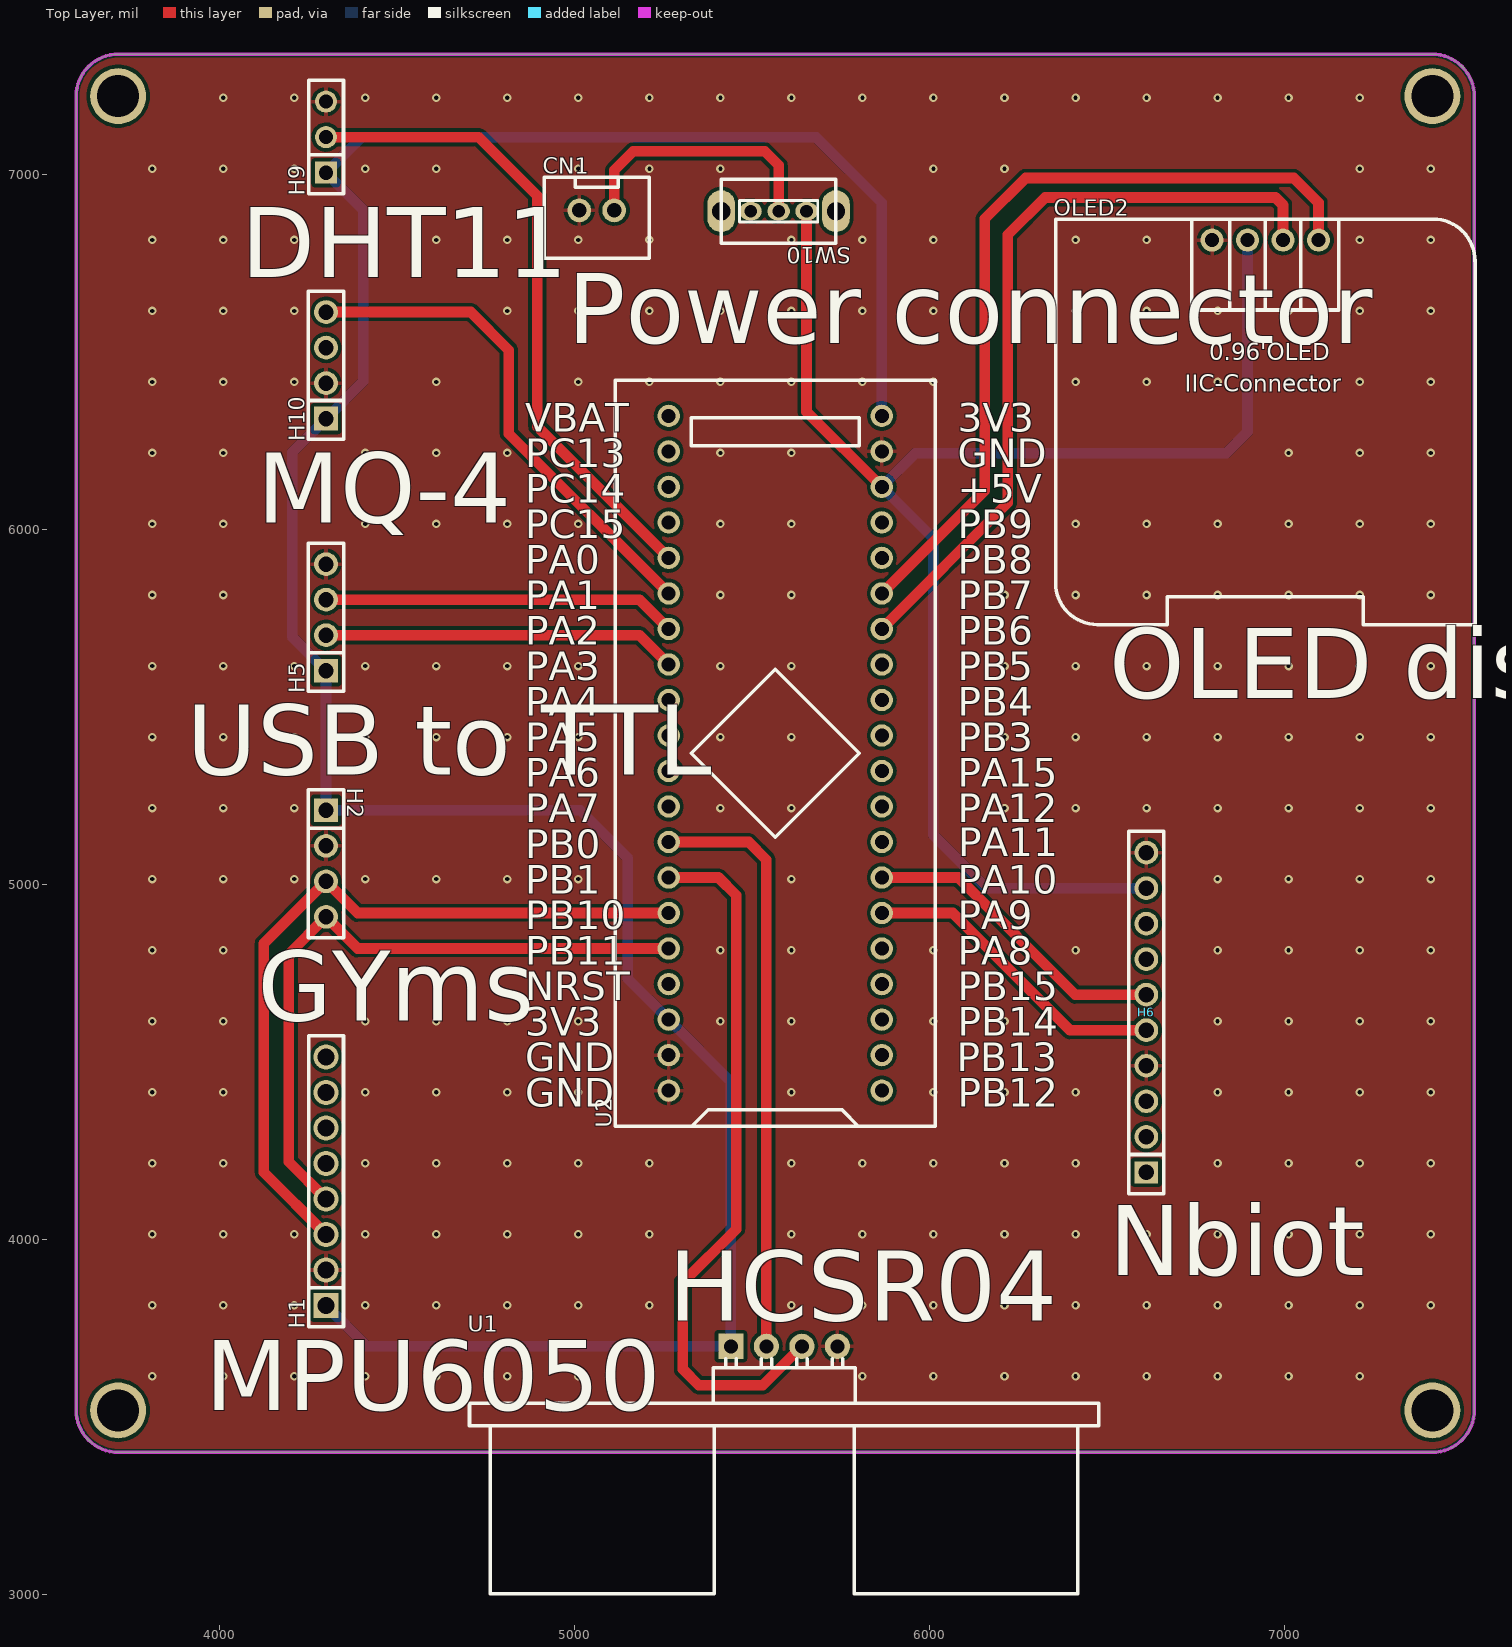
[diagram p0: Top Layer view]
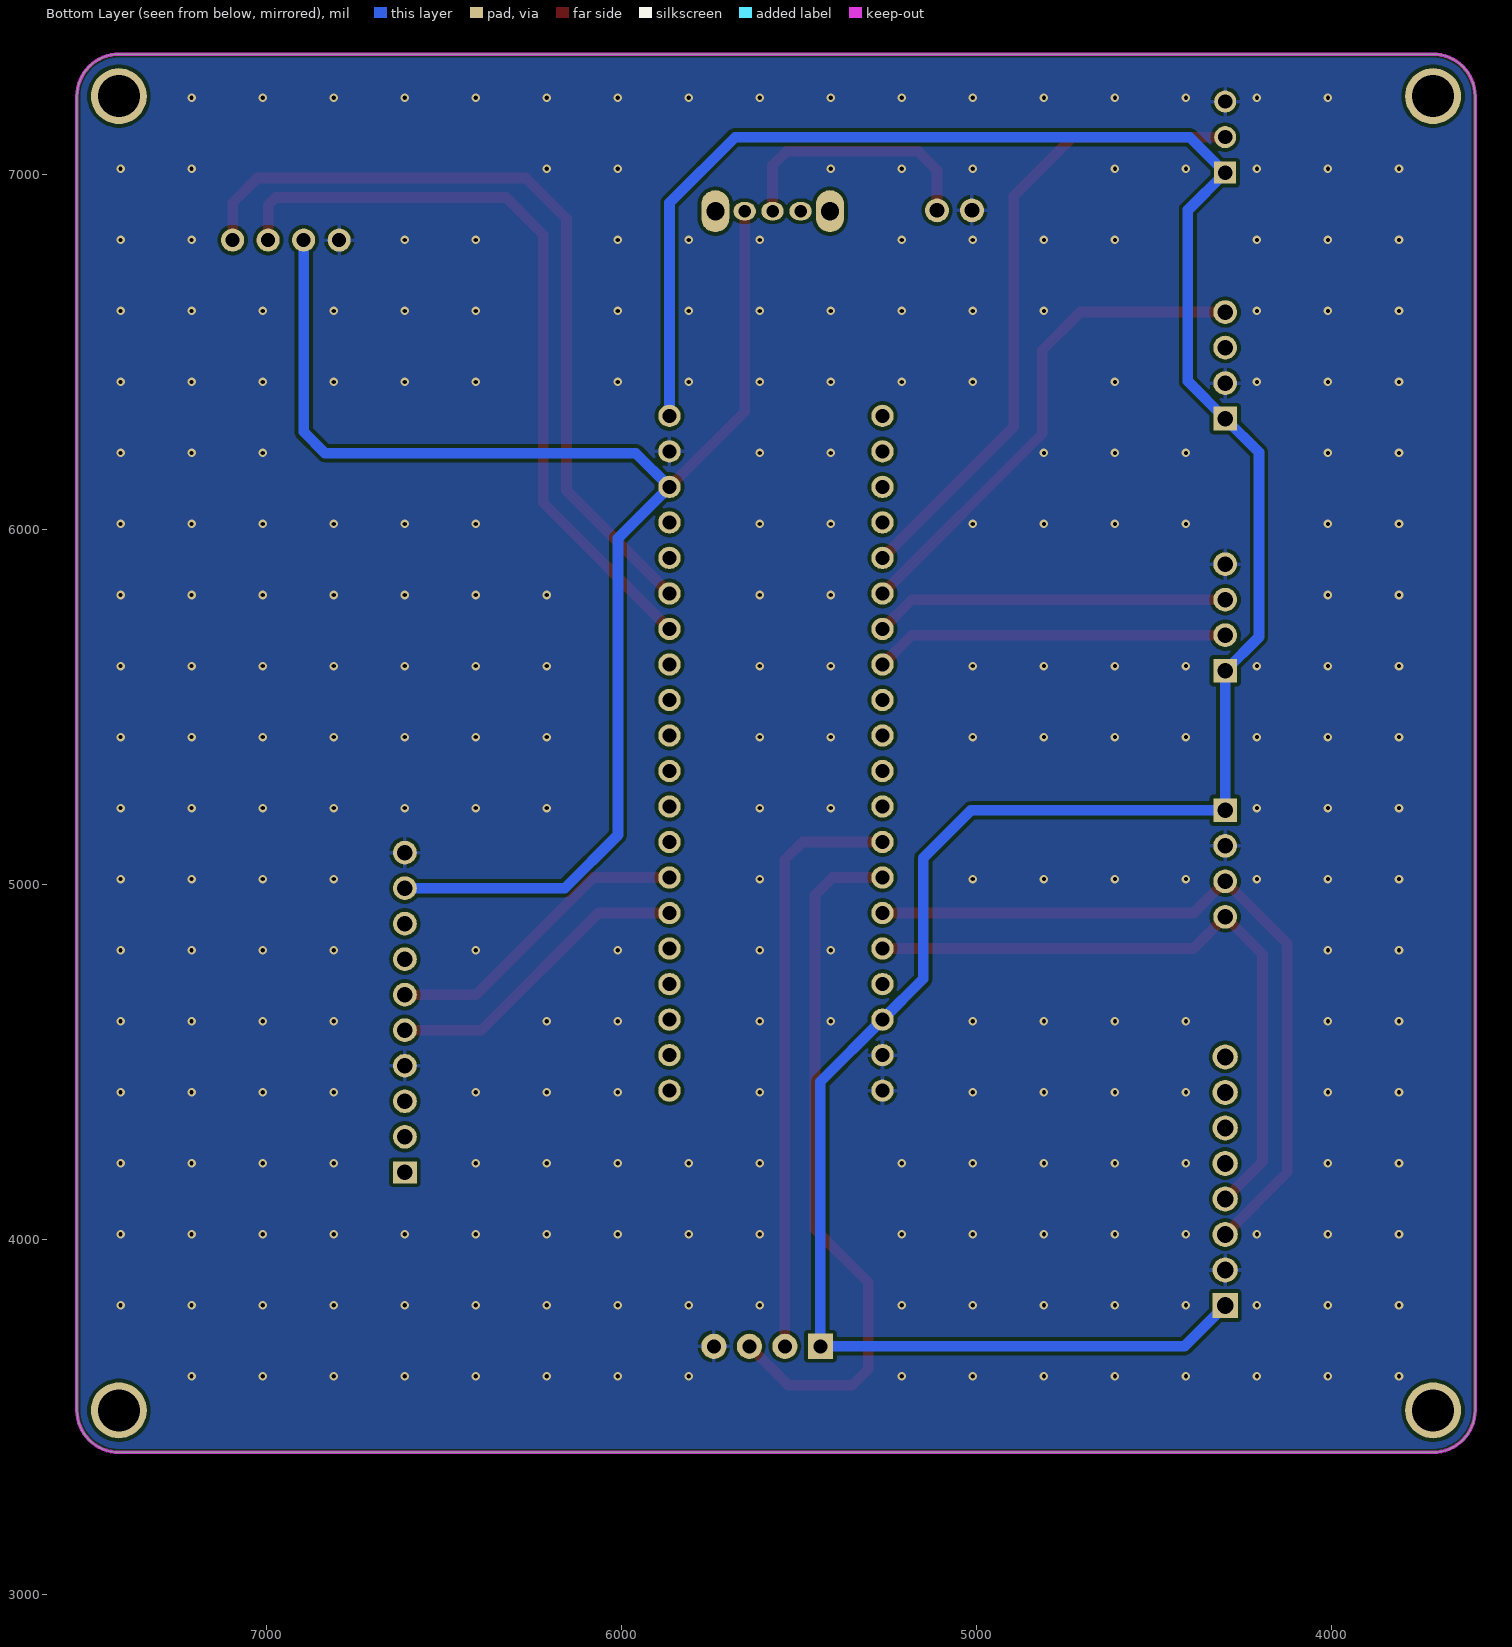
[diagram p1: Bottom Layer view, seen from below]
# Altium PCB MISC51645.pcbdoc
Units mil, origin at the board's own origin, x right, y up, seen from the top; angles counter-clockwise.
Board outline 3937.01 x 3937.01 mil, 2 copper layers (Top Layer, Bottom Layer), stack 62.206 mil thick; 11 components, 38 nets, 92 pads, 272 vias.

## Layer stack, top to bottom
Top Solder Mask Layer: solder mask 0.394, Dk 3.3
Top Layer: signal copper 1.379
Dielectric1: surface 59.449, FR4, Dk 4.5
Bottom Layer: signal copper 1.378
Bottom Solder Mask Layer: solder mask 0.394, Dk 3.3

## Board outline
3714.61,7337.72 ccw(c3714.61,7219.61) 3596.5,7219.61 3596.5,3518.82 ccw(c3714.61,3518.82) 3714.61,3400.71 7415.39,3400.71 ccw(c7415.39,3518.82) 7533.5,3518.82 7533.5,7219.61 ccw(c7415.39,7219.61) 7415.39,7337.72 3714.61,7337.72

## Design rules (kind name [scope] priority, off if disabled: settings)
BoardOutlineClearance copperThickness2oz_1 [All] p2 off: genericclearance=7.99 ignorepadtopadclearanceinfootprint=FALSE except(0: Arc-SplitContinuation Track-SplitContinuation SMDPad-SplitContinuation THPad-SplitContinuation Via-SplitContinuation Fill-SplitContinuation Region-SplitContinuation Poly-SplitContinuation Text-SplitContinuation Hole-SplitContinuation; 5.98: Arc-CutoutEdge Track-CutoutEdge SMDPad-CutoutEdge THPad-CutoutEdge Via-CutoutEdge Text-CutoutEdge; 6.9: Hole-OutlineEdge Hole-CutoutEdge; 10: Poly-OutlineEdge Poly-CutoutEdge; 11.81: Arc-OutlineEdge Track-OutlineEdge SMDPad-OutlineEdge THPad-OutlineEdge Via-OutlineEdge Fill-OutlineEdge Region-OutlineEdge Text-OutlineEdge Fill-CutoutEdge Region-CutoutEdge)
BoardOutlineClearance Plane_innerPlane_1 [All] p4 off: genericclearance=4.02 ignorepadtopadclearanceinfootprint=FALSE except(0: Arc-SplitContinuation Track-SplitContinuation SMDPad-SplitContinuation THPad-SplitContinuation Via-SplitContinuation Fill-SplitContinuation Region-SplitContinuation Poly-SplitContinuation Text-SplitContinuation Hole-SplitContinuation; 5.98: Arc-CutoutEdge Track-CutoutEdge SMDPad-CutoutEdge THPad-CutoutEdge Via-CutoutEdge Text-CutoutEdge; 6.9: Hole-OutlineEdge Hole-CutoutEdge; 10: Poly-OutlineEdge Poly-CutoutEdge; 11.81: Arc-OutlineEdge Track-OutlineEdge SMDPad-OutlineEdge THPad-OutlineEdge Via-OutlineEdge Fill-OutlineEdge Region-OutlineEdge Text-OutlineEdge Fill-CutoutEdge Region-CutoutEdge)
BoardOutlineClearance Copper_copperRegion_1 [All] p6 off: genericclearance=4.02 ignorepadtopadclearanceinfootprint=FALSE except(0: Arc-SplitContinuation Track-SplitContinuation SMDPad-SplitContinuation THPad-SplitContinuation Via-SplitContinuation Fill-SplitContinuation Region-SplitContinuation Poly-SplitContinuation Text-SplitContinuation Hole-SplitContinuation; 5.98: Arc-CutoutEdge Track-CutoutEdge SMDPad-CutoutEdge THPad-CutoutEdge Via-CutoutEdge Text-CutoutEdge; 6.9: Hole-OutlineEdge Hole-CutoutEdge; 10: Poly-OutlineEdge Poly-CutoutEdge; 11.81: Arc-OutlineEdge Track-OutlineEdge SMDPad-OutlineEdge THPad-OutlineEdge Via-OutlineEdge Fill-OutlineEdge Region-OutlineEdge Text-OutlineEdge Fill-CutoutEdge Region-CutoutEdge)
BoardOutlineClearance Copper_copperRegion_copperThickness1oz_1 [All] p8 off: genericclearance=4.02 ignorepadtopadclearanceinfootprint=FALSE except(0: Arc-SplitContinuation Track-SplitContinuation SMDPad-SplitContinuation THPad-SplitContinuation Via-SplitContinuation Fill-SplitContinuation Region-SplitContinuation Poly-SplitContinuation Text-SplitContinuation Hole-SplitContinuation; 5.98: Arc-CutoutEdge Track-CutoutEdge SMDPad-CutoutEdge THPad-CutoutEdge Via-CutoutEdge Text-CutoutEdge; 6.9: Hole-OutlineEdge Hole-CutoutEdge; 10: Poly-OutlineEdge Poly-CutoutEdge; 11.81: Arc-OutlineEdge Track-OutlineEdge SMDPad-OutlineEdge THPad-OutlineEdge Via-OutlineEdge Fill-OutlineEdge Region-OutlineEdge Text-OutlineEdge Fill-CutoutEdge Region-CutoutEdge)
BoardOutlineClearance Copper_copperRegion_Copper_copperRegion_1 [All] p10 off: genericclearance=4.02 ignorepadtopadclearanceinfootprint=FALSE except(0: Arc-SplitContinuation Track-SplitContinuation SMDPad-SplitContinuation THPad-SplitContinuation Via-SplitContinuation Fill-SplitContinuation Region-SplitContinuation Poly-SplitContinuation Text-SplitContinuation Hole-SplitContinuation; 5.98: Arc-CutoutEdge Track-CutoutEdge SMDPad-CutoutEdge THPad-CutoutEdge Via-CutoutEdge Text-CutoutEdge; 6.9: Hole-OutlineEdge Hole-CutoutEdge; 10: Poly-OutlineEdge Poly-CutoutEdge; 11.81: Arc-OutlineEdge Track-OutlineEdge SMDPad-OutlineEdge THPad-OutlineEdge Via-OutlineEdge Fill-OutlineEdge Region-OutlineEdge Text-OutlineEdge Fill-CutoutEdge Region-CutoutEdge)
BoardOutlineClearance copperThickness1oz_1 [All] p12: genericclearance=4.02 ignorepadtopadclearanceinfootprint=FALSE except(0: Arc-SplitContinuation Track-SplitContinuation SMDPad-SplitContinuation THPad-SplitContinuation Via-SplitContinuation Fill-SplitContinuation Region-SplitContinuation Poly-SplitContinuation Text-SplitContinuation Hole-SplitContinuation; 5.98: Arc-CutoutEdge Track-CutoutEdge SMDPad-CutoutEdge THPad-CutoutEdge Via-CutoutEdge Text-CutoutEdge; 6.9: Hole-OutlineEdge Hole-CutoutEdge; 10: Poly-OutlineEdge Poly-CutoutEdge; 11.81: Arc-OutlineEdge Track-OutlineEdge SMDPad-OutlineEdge THPad-OutlineEdge Via-OutlineEdge Fill-OutlineEdge Region-OutlineEdge Text-OutlineEdge Fill-CutoutEdge Region-CutoutEdge)
Clearance copperThickness2oz [All] p1 off: gap=7.99 ignorepadtopadclearanceinfootprint=FALSE except(5.98: SMDPad-Track SMDPad-SMDPad THPad-Track SMDPad-THPad THPad-THPad Track-Via SMDPad-Via THPad-Via Via-Via Fill-SMDPad Region-SMDPad Fill-THPad Region-THPad Fill-Via Region-Via Fill-Fill Fill-Region Region-Region Arc-Track Arc-SMDPad Arc-THPad Arc-Via Fill-Arc Region-Arc Arc-Arc Text-Track SMDPad-Text Text-THPad Text-Via Fill-Text Region-Text Arc-Text Text-Text; 6.9: Hole-Track Hole-SMDPad Hole-THPad Hole-Via Fill-Hole Region-Hole Hole-Arc Hole-Text; 10: Poly-Track Poly-SMDPad Poly-THPad Poly-Via Poly-Fill Poly-Region Poly-Poly Poly-Arc Poly-Text Poly-Hole; 11.81: Fill-Track Region-Track)
Clearance Plane_innerPlane [All] p3 off: gap=4.02 ignorepadtopadclearanceinfootprint=FALSE except(5.98: SMDPad-Track SMDPad-SMDPad THPad-Track SMDPad-THPad THPad-THPad Track-Via SMDPad-Via THPad-Via Via-Via Fill-SMDPad Region-SMDPad Fill-THPad Region-THPad Fill-Via Region-Via Fill-Fill Fill-Region Region-Region Arc-Track Arc-SMDPad Arc-THPad Arc-Via Fill-Arc Region-Arc Arc-Arc Text-Track SMDPad-Text Text-THPad Text-Via Fill-Text Region-Text Arc-Text Text-Text; 6.9: Hole-Track Hole-SMDPad Hole-THPad Hole-Via Fill-Hole Region-Hole Hole-Arc Hole-Text; 10: Poly-Track Poly-SMDPad Poly-THPad Poly-Via Poly-Fill Poly-Region Poly-Poly Poly-Arc Poly-Text Poly-Hole; 11.81: Fill-Track Region-Track)
Clearance Copper_copperRegion [All] p5 off: gap=4.02 ignorepadtopadclearanceinfootprint=FALSE except(5.98: SMDPad-Track SMDPad-SMDPad THPad-Track SMDPad-THPad THPad-THPad Track-Via SMDPad-Via THPad-Via Via-Via Fill-SMDPad Region-SMDPad Fill-THPad Region-THPad Fill-Via Region-Via Fill-Fill Fill-Region Region-Region Arc-Track Arc-SMDPad Arc-THPad Arc-Via Fill-Arc Region-Arc Arc-Arc Text-Track SMDPad-Text Text-THPad Text-Via Fill-Text Region-Text Arc-Text Text-Text; 6.9: Hole-Track Hole-SMDPad Hole-THPad Hole-Via Fill-Hole Region-Hole Hole-Arc Hole-Text; 10: Poly-Track Poly-SMDPad Poly-THPad Poly-Via Poly-Fill Poly-Region Poly-Poly Poly-Arc Poly-Text Poly-Hole; 11.81: Fill-Track Region-Track)
Clearance Copper_copperRegion_copperThickness1oz [All] p7 off: gap=4.02 ignorepadtopadclearanceinfootprint=FALSE except(5.98: SMDPad-Track SMDPad-SMDPad THPad-Track SMDPad-THPad THPad-THPad Track-Via SMDPad-Via THPad-Via Via-Via Fill-SMDPad Region-SMDPad Fill-THPad Region-THPad Fill-Via Region-Via Fill-Fill Fill-Region Region-Region Arc-Track Arc-SMDPad Arc-THPad Arc-Via Fill-Arc Region-Arc Arc-Arc Text-Track SMDPad-Text Text-THPad Text-Via Fill-Text Region-Text Arc-Text Text-Text; 6.9: Hole-Track Hole-SMDPad Hole-THPad Hole-Via Fill-Hole Region-Hole Hole-Arc Hole-Text; 10: Poly-Track Poly-SMDPad Poly-THPad Poly-Via Poly-Fill Poly-Region Poly-Poly Poly-Arc Poly-Text Poly-Hole; 11.81: Fill-Track Region-Track)
Clearance Copper_copperRegion_Copper_copperRegion [All] p9 off: gap=4.02 ignorepadtopadclearanceinfootprint=FALSE except(5.98: SMDPad-Track SMDPad-SMDPad THPad-Track SMDPad-THPad THPad-THPad Track-Via SMDPad-Via THPad-Via Via-Via Fill-SMDPad Region-SMDPad Fill-THPad Region-THPad Fill-Via Region-Via Fill-Fill Fill-Region Region-Region Arc-Track Arc-SMDPad Arc-THPad Arc-Via Fill-Arc Region-Arc Arc-Arc Text-Track SMDPad-Text Text-THPad Text-Via Fill-Text Region-Text Arc-Text Text-Text; 6.9: Hole-Track Hole-SMDPad Hole-THPad Hole-Via Fill-Hole Region-Hole Hole-Arc Hole-Text; 10: Poly-Track Poly-SMDPad Poly-THPad Poly-Via Poly-Fill Poly-Region Poly-Poly Poly-Arc Poly-Text Poly-Hole; 11.81: Fill-Track Region-Track)
Clearance copperThickness1oz [All] p11: gap=4.02 ignorepadtopadclearanceinfootprint=FALSE except(5.98: SMDPad-Track SMDPad-SMDPad THPad-Track SMDPad-THPad THPad-THPad Track-Via SMDPad-Via THPad-Via Via-Via Fill-SMDPad Region-SMDPad Fill-THPad Region-THPad Fill-Via Region-Via Fill-Fill Fill-Region Region-Region Arc-Track Arc-SMDPad Arc-THPad Arc-Via Fill-Arc Region-Arc Arc-Arc Text-Track SMDPad-Text Text-THPad Text-Via Fill-Text Region-Text Arc-Text Text-Text; 6.9: Hole-Track Hole-SMDPad Hole-THPad Hole-Via Fill-Hole Region-Hole Hole-Arc Hole-Text; 10: Poly-Track Poly-SMDPad Poly-THPad Poly-Via Poly-Fill Poly-Region Poly-Poly Poly-Arc Poly-Text Poly-Hole; 11.81: Fill-Track Region-Track)
DiffPairsRouting differentialPair [All] p1: maxlimit=6 minlimit=6 mostfreqgap=6 toplayer_minwidth=5 toplayer_prefwidth=10 toplayer_maxwidth=100 toplayer_mingap=6 toplayer_prefgap=6 toplayer_maxgap=6 bottomlayer_minwidth=5 bottomlayer_prefwidth=10 bottomlayer_maxwidth=100 bottomlayer_mingap=6 bottomlayer_prefgap=6 bottomlayer_maxgap=6 maxuncoupledlength=10
HoleToHoleClearance otherClearance [All] p1: gap=11.81 allowstackedmicrovias=TRUE
Length netLength [All] p1: minlimit=0 maxlimit=0
PasteMaskExpansion pasteMaskExpansion [All] p1: expansion=0
PlaneConnect innerPlane [All] p1: planeconnectstyle=Relief reliefexpansion=20 reliefentries=4 reliefconductorwidth=10 reliefairgap=10
PolygonConnect copperRegion_copperThickness1oz [All] p1 off: connectstyle=Relief reliefconductorwidth=10 reliefentries=4 polygonreliefangle="90 Angle" airgapwidth=10 via.connectstyle=Relief via.reliefconductorwidth=10 via.reliefentries=4 via.polygonreliefangle="90 Angle" via.airgapwidth=10
PolygonConnect copperRegion_Copper_copperRegion [All] p2 off: connectstyle=Relief reliefconductorwidth=10 reliefentries=4 polygonreliefangle="90 Angle" airgapwidth=10 via.connectstyle=Relief via.reliefconductorwidth=10 via.reliefentries=4 via.polygonreliefangle="90 Angle" via.airgapwidth=10
PolygonConnect copperRegion [All] p3: connectstyle=Relief reliefconductorwidth=10 reliefentries=4 polygonreliefangle="90 Angle" airgapwidth=10 via.connectstyle=Relief via.reliefconductorwidth=10 via.reliefentries=4 via.polygonreliefangle="90 Angle" via.airgapwidth=10
RoutingVias viaSize [All] p1: holewidth=12.01 width=24.02 viastyle="Through Hole" minholewidth=11.81 minwidth=19.68 maxholewidth=248.03 maxwidth=393.7
SolderMaskExpansion solderMaskExpansion [IsVia] p1: expansion=-1000 istentingtop=TRUE
SolderMaskExpansion solderMaskExpansion [All] p2: expansion=2 istentingtop=FALSE
Width copperThickness2oz_2 [All] p1 off: maxlimit=100 minlimit=8 preferedwidth=10
Width copperThickness1oz_2 [All] p2: maxlimit=100 minlimit=5 preferedwidth=10

## Components (designator, comment, footprint, x,y, rotation, side; value= is the part's Value field where it differs from the comment)
CN1 "XH2.54*2P_straight" CONN-TH_2P-P2.50-XH2.54-2P 5062.33,6897.87 r0 top
H1 "" HDR-TH_8P-P2.54-V-F-1 4300,4164.01 r90 top
H2 "" HDR-TH_4P-P2.54-V-F 4300,5058.47 r270 top
H5 "" HDR-TH_4P-P2.54-V-F 4300,5751.66 r90 top
H6 "" HDR-TH_10P-P2.54-V-F 6610,4639.21 r90 top
H9 "" HDR-TH_3P-P2.54-V-F 4300,7104.21 r90 top
H10 "" HDR-TH_4P-P2.54-V-F 4300,6461.54 r90 top
OLED2 "" 0.96OLED_4P 6945,6814.21 r0 top
SW10 "" 拨动开关 5579.64,6895.56 r180 top
U1 "HC-SR04" TH_HC-SR04V 5590,3699.21 r0 top
U2 "STM32F103C8T6-Card" CONN-TH_L53.3-W22.9_STM32F103C8T6-CARD 5565,5369.21 r90 top

## Footprints (in the part's own frame and the unit in brackets; to place one, negate y for a bottom-side part, rotate by r counter-clockwise, add the part's x,y. Pads: shape width x height; smd on the part's side, far side on the other; paste and mask are expansions set on the pad)
0.96OLED_4P [mm]
  round 1.65 hole 1 copper offset 0,0: 1(-3.81,-0.001) 2(-1.27,0.002) 3(1.27,0.002) 4(3.81,0.002)
  silkscreen extent -15,-27.5 15,1.5
CONN-TH_2P-P2.50-XH2.54-2P [mm]
  round 1.7 hole 1.05 paste+0 mask+0.05: 1(1.25,0) 2(-1.25,0)
  silkscreen extent -3.75,-3.42 3.75,2.37
CONN-TH_L53.3-W22.9_STM32F103C8T6-CARD [mm]
  round 1.6 hole 1: 1(-24.13,-7.62) 2(-21.59,-7.62) 3(-19.05,-7.62) 4(-16.51,-7.62) 5(-13.97,-7.62) 6(-11.43,-7.62) 7(-8.89,-7.62) 8(-6.35,-7.62) 9(-3.81,-7.62) 10(-1.27,-7.62) 11(1.27,-7.62) 12(3.81,-7.62) 13(6.35,-7.62) 14(8.89,-7.62) 15(11.43,-7.62) 16(13.97,-7.62) 17(16.51,-7.62) 18(19.05,-7.62) 19(21.59,-7.62) 20(24.13,-7.62) 21(24.13,7.62) 22(21.59,7.62) 23(19.05,7.62) 24(16.51,7.62) 25(13.97,7.62) 26(11.43,7.62) 27(8.89,7.62) 28(6.35,7.62) 29(3.81,7.62) 30(1.27,7.62) 31(-1.27,7.62) 32(-3.81,7.62) 33(-6.35,7.62) 34(-8.89,7.62) 35(-11.43,7.62) 36(-13.97,7.62) 37(-16.51,7.62) 38(-19.05,7.62) 39(-21.59,7.62) 40(-24.13,7.62)
  silkscreen extent -26.67,-11.43 26.67,11.43
HDR-TH_3P-P2.54-V-F [mil]
  rect 62x62 hole 40.16: 1(-100,0)
  round 62 hole 40.16: 2(0,0) 3(100,0)
  silkscreen extent -160,-49 160,49
HDR-TH_4P-P2.54-V-F [mm]
  rect 1.7x1.7 hole 1.1: 1(-3.81,0)
  round 1.7 hole 1.1: 2(-1.27,0) 3(1.27,0) 4(3.81,0)
  silkscreen extent -5.29,-1.27 5.29,1.27
HDR-TH_8P-P2.54-V-F-1 [mm]
  rect 1.8x1.8 hole 1.2: 1(-8.89,0)
  round 1.8 hole 1.2: 2(-6.35,0) 3(-3.81,0) 4(-1.27,0) 5(1.27,0) 6(3.81,0) 7(6.35,0) 8(8.89,0)
  silkscreen extent -10.41,-1.25 10.41,1.25
HDR-TH_10P-P2.54-V-F [mm]
  rect 1.575x1.7 hole 1.1: 1(-11.43,0)
  round 1.7 hole 1.1: 2(-8.89,0) 3(-6.35,0) 4(-3.81,0) 5(-1.27,0) 6(1.27,0) 7(3.81,0) 8(6.35,0) 9(8.89,0) 10(11.43,0)
  silkscreen extent -12.95,-1.25 12.95,1.25
TH_HC-SR04V [mm]
  rect 1.8x1.8 hole 1.001: 1(-3.81,0)
  round 1.8 hole 1.001: 2(-1.27,0) 3(1.27,0) 4(3.81,0)
  silkscreen extent -22.5,-17.7 22.5,-0.89
拨动开关 [mil]
  oval 63x51.2 hole 35.4 paste+0 mask+2: 1(-73.4,0) 2(5,0) 3(84,0)
  oval 78.7x118.1 hole 51.2 paste+0 mask+2: 4(166.7,0) 5(-156.1,0)
  silkscreen extent -156,-90 167,90

## Free pads (board coordinates)
  round 157.48 hole 118.11: 1(3714.61,7219.61) 1(3714.61,3518.82) 1(7415.39,7219.61) 1(7415.39,3518.82)

## Via types
v1: diameter 24.02, hole 12, Top Layer to Bottom Layer, 272 vias

## Nets (pads, with @x,y where several pads share a name; then routed paths per layer and width w, separated by ;. In a path a pad name is that pad's centre, name@x,y a point inside that pad or via, vN(x,y) a via of type N, cw(c..) or ccw(c..) an arc to the next point about the centre after c; other vN are vias at no path point)
$1N17202: CN1.1 SW10.2 | length 743.5
  Top Layer w30: CN1.1 5111.54,7010.76 5165,7064.21 5535,7064.21 5574.64,7024.58 SW10.2
+5V: H6.9 OLED2.2 SW10.1 U2.18 | length 4200.6
  Top Layer w30: SW10.1 5653.04,6331.18 U2.18
  Bottom Layer w30: H6.9 6160,4989.21 6010,5139.21 6010,5974.21 U2.18 5960,6214.21 6835,6214.21 6895,6274.21 OLED2.2
GND: CN1.2 H1.2 H2.2 H5.4 H6.4 H6.10 H9.3 H10.2 OLED2.1 U1.4 U2.19 U2.39 U2.40
  other v1: 3810.6,3614.81 4010.6,3614.81 4210.6,3614.81 4410.6,3614.81 4610.6,3614.81 4810.6,3614.81 5010.6,3614.81 5210.6,3614.81 5810.6,3614.81 6010.6,3614.81 6210.6,3614.81 6410.6,3614.81 6610.6,3614.81 6810.6,3614.81 7010.6,3614.81 7210.6,3614.81 3810.6,3814.81 4010.6,3814.81 4210.6,3814.81 4410.6,3814.81 4610.6,3814.81 4810.6,3814.81 5010.6,3814.81 5210.6,3814.81 5610.6,3814.81 5810.6,3814.81 6010.6,3814.81 6210.6,3814.81 6410.6,3814.81 6610.6,3814.81 6810.6,3814.81 7010.6,3814.81 7210.6,3814.81 7410.6,3814.81 3810.6,4014.81 4010.6,4014.81 4210.6,4014.81 4410.6,4014.81 4610.6,4014.81 4810.6,4014.81 5010.6,4014.81 5210.6,4014.81 5610.6,4014.81 5810.6,4014.81 6010.6,4014.81 6210.6,4014.81 6410.6,4014.81 6610.6,4014.81 6810.6,4014.81 7010.6,4014.81 7210.6,4014.81 7410.6,4014.81 3810.6,4214.81 4010.6,4214.81 4410.6,4214.81 4610.6,4214.81 4810.6,4214.81 5010.6,4214.81 5210.6,4214.81 5610.6,4214.81 5810.6,4214.81 6010.6,4214.81 6210.6,4214.81 6410.6,4214.81 6810.6,4214.81 7010.6,4214.81 7210.6,4214.81 7410.6,4214.81 3810.6,4414.81 4010.6,4414.81 4410.6,4414.81 4610.6,4414.81 4810.6,4414.81 5010.6,4414.81 5610.6,4414.81 6010.6,4414.81 6210.6,4414.81 6410.6,4414.81 6810.6,4414.81 7010.6,4414.81 7210.6,4414.81 7410.6,4414.81 3810.6,4614.81 4010.6,4614.81 4410.6,4614.81 4610.6,4614.81 4810.6,4614.81 5010.6,4614.81 5410.6,4614.81 5610.6,4614.81 6010.6,4614.81 6210.6,4614.81 6810.6,4614.81 7010.6,4614.81 7210.6,4614.81 7410.6,4614.81 3810.6,4814.81 4010.6,4814.81 5410.6,4814.81 5610.6,4814.81 6010.6,4814.81 6410.6,4814.81 6810.6,4814.81 7010.6,4814.81 7210.6,4814.81 7410.6,4814.81 3810.6,5014.81 4010.6,5014.81 4210.6,5014.81 4410.6,5014.81 4610.6,5014.81 4810.6,5014.81 5010.6,5014.81 5610.6,5014.81 6810.6,5014.81 7010.6,5014.81 7210.6,5014.81 7410.6,5014.81 3810.6,5214.81 4010.6,5214.81 4210.6,5214.81 5410.6,5214.81 5610.6,5214.81 6210.6,5214.81 6410.6,5214.81 6610.6,5214.81 6810.6,5214.81 7010.6,5214.81 7210.6,5214.81 7410.6,5214.81 3810.6,5414.81 4010.6,5414.81 4210.6,5414.81 4410.6,5414.81 4610.6,5414.81 4810.6,5414.81 5010.6,5414.81 5410.6,5414.81 5610.6,5414.81 6210.6,5414.81 6410.6,5414.81 6610.6,5414.81 6810.6,5414.81 7010.6,5414.81 7210.6,5414.81 7410.6,5414.81 3810.6,5614.81 4010.6,5614.81 4210.6,5614.81 4410.6,5614.81 4610.6,5614.81 4810.6,5614.81 5010.6,5614.81 5410.6,5614.81 5610.6,5614.81 6210.6,5614.81 6410.6,5614.81 6610.6,5614.81 6810.6,5614.81 7010.6,5614.81 7210.6,5614.81 7410.6,5614.81 3810.6,5814.81 4010.6,5814.81 5410.6,5814.81 5610.6,5814.81 6210.6,5814.81 6410.6,5814.81 6610.6,5814.81 6810.6,5814.81 7010.6,5814.81 7210.6,5814.81 7410.6,5814.81 3810.6,6014.81 4010.6,6014.81 4410.6,6014.81 4610.6,6014.81 4810.6,6014.81 5010.6,6014.81 5410.6,6014.81 5610.6,6014.81 6410.6,6014.81 6610.6,6014.81 6810.6,6014.81 7010.6,6014.81 7210.6,6014.81 7410.6,6014.81 3810.6,6214.81 4010.6,6214.81 4410.6,6214.81 4610.6,6214.81 4810.6,6214.81 5410.6,6214.81 5610.6,6214.81 7010.6,6214.81 7210.6,6214.81 7410.6,6214.81 3810.6,6414.81 4010.6,6414.81 4210.6,6414.81 4610.6,6414.81 5010.6,6414.81 5210.6,6414.81 5410.6,6414.81 5610.6,6414.81 5810.6,6414.81 6010.6,6414.81 6410.6,6414.81 6610.6,6414.81 6810.6,6414.81 7010.6,6414.81 7210.6,6414.81 7410.6,6414.81 3810.6,6614.81 4010.6,6614.81 4210.6,6614.81 4810.6,6614.81 5010.6,6614.81 5210.6,6614.81 5410.6,6614.81 5610.6,6614.81 5810.6,6614.81 6010.6,6614.81 6410.6,6614.81 6610.6,6614.81 6810.6,6614.81 7010.6,6614.81 7210.6,6614.81 7410.6,6614.81 3810.6,6814.81 4010.6,6814.81 4210.6,6814.81 4610.6,6814.81 4810.6,6814.81 5010.6,6814.81 5210.6,6814.81 5610.6,6814.81 5810.6,6814.81 6010.6,6814.81 6410.6,6814.81 6610.6,6814.81 7210.6,6814.81 7410.6,6814.81 3810.6,7014.81 4010.6,7014.81 4210.6,7014.81 4410.6,7014.81 4610.6,7014.81 5010.6,7014.81 5210.6,7014.81 5410.6,7014.81 6010.6,7014.81 6210.6,7014.81 7210.6,7014.81 7410.6,7014.81 4010.6,7214.81 4210.6,7214.81 4410.6,7214.81 4610.6,7214.81 4810.6,7214.81 5010.6,7214.81 5210.6,7214.81 5410.6,7214.81 5610.6,7214.81 5810.6,7214.81 6010.6,7214.81 6210.6,7214.81 6410.6,7214.81 6610.6,7214.81 6810.6,7214.81 7010.6,7214.81 7210.6,7214.81
NRST: U2.37
PA0: H9.2 U2.25 | length 1836.6
  Top Layer w30: H9.2 4730,7104.21 4895,6939.21 4895,6289.21 U2.25
PA1: H10.4 U2.26 | length 1430.9
  Top Layer w30: H10.4 4707.67,6611.54 4815,6504.21 4815,6269.21 U2.26
PA2: H5.3 U2.27 | length 999.1
  Top Layer w30: H5.3 5182.56,5801.66 U2.27
PA3: H5.2 U2.28 | length 999.1
  Top Layer w30: H5.2 5182.56,5701.66 U2.28
PA4: U2.29
PA5: U2.30
PA6: U2.31
PA7: U2.32
PA8: U2.5
PA9: H6.5 U2.6 | length 881.7
  Top Layer w30: U2.6 6065,4919.21 6395,4589.21 H6.5
PA10: H6.6 U2.7 | length 881.7
  Top Layer w30: U2.7 6080,5019.21 6410,4689.21 H6.6
PA11: U2.8
PA12: U2.9
PA15: U2.10
PB0: U1.2 U2.33 | length 1665.7
  Top Layer w30: U2.33 5490,5119.21 5540,5069.21 U1.2
PB1: U1.3 U2.34 | length 2007
  Top Layer w30: U2.34 5405,5019.21 5455,4969.21 5455,4029.21 5305,3879.21 5305,3634.21 5350,3589.21 5530,3589.21 U1.3
PB3: U2.11
PB4: U2.12
PB5: U2.13
PB6: OLED2.3 U2.14 | length 2183.1
  Top Layer w30: U2.14 6220,6074.22 6220,6829.21 6325,6934.21 6973.79,6934.21 6995,6913 OLED2.3
PB7: OLED2.4 U2.15 | length 2296.7
  Top Layer w30: U2.15 6155,6109.22 6155,6874.21 6270,6989.21 7025,6989.21 7095,6919.21 OLED2.4
PB8: U2.16
PB9: U2.17
PB10: H1.3 H2.3 U2.35 | length 2141.4
  Top Layer w30: H1.3 4125,4189.01 4125,4833.47 H2.3 4389.26,4919.21 U2.35
PB11: H1.4 H2.4 U2.36 | length 1883.4
  Top Layer w30: H1.4 4195,4219.01 4195,4803.47 H2.4 4389.26,4819.21 U2.36
PB12: U2.1
PB13: U2.2
PB14: U2.3
PB15: U2.4
PC13: U2.22
PC14: U2.23
PC15: U2.24
VBAT: U2.21
VCC: H1.1 H2.1 H5.1 H9.1 H10.1 U1.1 U2.20 U2.38 | length 7832.8
  Bottom Layer w30: H1.1 4414.8,3699.21 U1.1 5440,4444.21 U2.38 5150,4734.21 5150,5074.21 5015.74,5208.47 H2.1 H5.1 4205,5696.66 4205,6216.54 H10.1 4405,6416.54 4405,6899.21 H9.1 4400,7104.21 5680,7104.21 5865,6919.21 U2.20
pads on no net: H1.5 H1.6 H1.7 H1.8 H6.1 H6.2 H6.3 H6.7 H6.8 H10.3 SW10.3 SW10.4 SW10.5

## Polygon pours and split planes (outlines as drawn)
GND on Bottom Layer (solid, remove dead copper, pour order 2): 3525,7459.21 3525,3294.21 7700,3294.21 7700,7459.21
GND on Top Layer (solid, remove dead copper, pour order 2): 3000,7629.21 3000,3214.21 7930,3214.21 7930,7629.21

## Keep-outs
Board Outline Layer:
  the board outline again, w10

## Silkscreen, mask and mechanical layers (free items; w line width, h text height)
Top Silkscreen Layer:
  text "DHT11" at 4061.39,6709.71 h196.85
  text "Power connector" at 4980,6524.21 h196.85
  text "VBAT" at 4860.95,6274.21 h80
  text "3V3" at 6079.16,6274.21 h80
  text "PC13" at 4860.95,6174.21 h80
  text "GND" at 6079.16,6174.21 h80
  text "PC14" at 4860.95,6074.21 h80
  text "+5V" at 6079.16,6074.21 h80
  text "MQ-4" at 4105.98,6018.31 h196.85
  text "PC15" at 4860.95,5974.21 h80
  text "PB9" at 6079.16,5974.21 h80
  text "PA0" at 4860.95,5874.21 h80
  text "PB8" at 6079.16,5874.21 h80
  text "PA1" at 4860.95,5774.21 h80
  text "PB7" at 6079.16,5774.21 h80
  text "PA2" at 4860.95,5674.21 h80
  text "PB6" at 6079.16,5674.21 h80
  text "PA3" at 4860.95,5574.21 h80
  text "PB5" at 6079.16,5574.21 h80
  text "OLED display" at 6505,5524.21 h196.85
  text "PA4" at 4860.95,5474.21 h80
  text "PB4" at 6079.16,5474.21 h80
  text "PA5" at 4860.95,5374.21 h80
  text "PB3" at 6079.16,5374.21 h80
  text "USB to TTL" at 3908.24,5308.43 h196.85
  text "PA6" at 4860.95,5274.21 h80
  text "PA15" at 6079.16,5274.21 h80
  text "PA7" at 4860.95,5174.21 h80
  text "PA12" at 6079.16,5174.21 h80
  text "PA11" at 6080.95,5079.21 h80
  text "PB0" at 4860.95,5074.21 h80
  text "PB1" at 4860.95,4974.21 h80
  text "PA10" at 6079.16,4974.21 h80
  text "PB10" at 4860.95,4874.21 h80
  text "PA9" at 6079.16,4874.21 h80
  text "PB11" at 4860.95,4774.21 h80
  text "PA8" at 6079.16,4774.21 h80
  text "NRST" at 4860.95,4674.21 h80
  text "PB15" at 6079.16,4674.21 h80
  text "GYms" at 4108.07,4615.54 h196.85
  text "3V3" at 4860.95,4574.21 h80
  text "PB14" at 6079.16,4574.21 h80
  text "GND" at 4860.95,4474.21 h80
  text "PB13" at 6075.95,4474.21 h80
  text "GND" at 4860.95,4374.21 h80
  text "PB12" at 6079.16,4374.21 h80
  text "Nbiot" at 6505,3899.21 h196.85
  text "HCSR04" at 5264.72,3770.79 h196.85
  text "MPU6050" at 3959.69,3519.21 h196.85